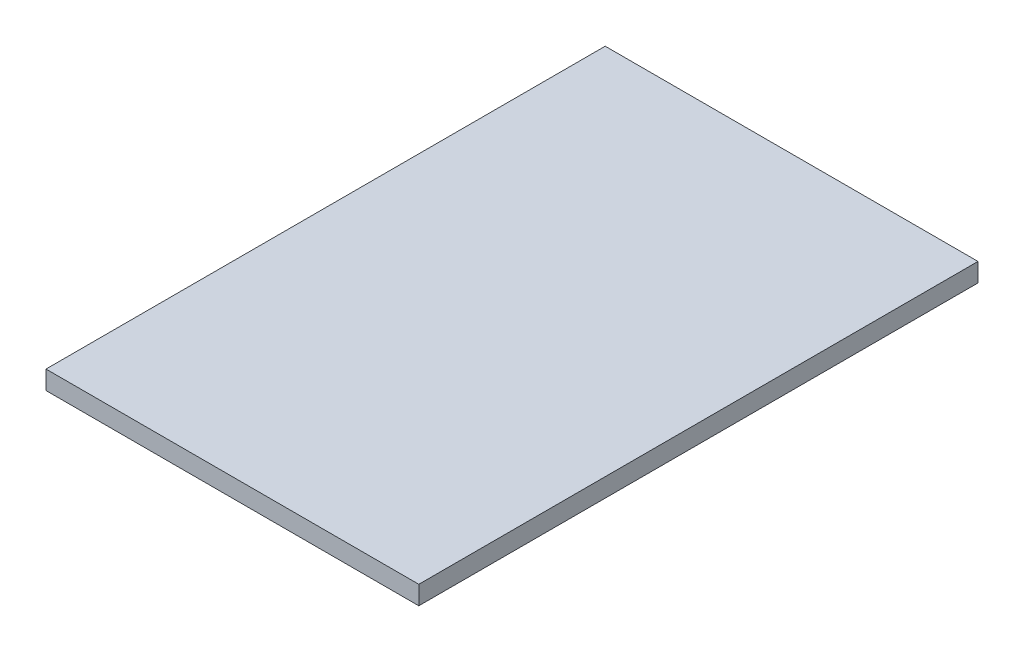
from build123d import *

# Parameters (mm, degrees)
SKETCH2_W           = 200
SKETCH2_H           = 300
BOSS_EXTRUDE1_DEPTH = 10


with BuildPart() as part:
    # Sketch2 → Boss-Extrude1 (new body)
    with BuildSketch(Plane(origin=(0, 0, 0), x_dir=(1, 0, 0), z_dir=(0, 1, 0))):
        Rectangle(SKETCH2_W, SKETCH2_H)
    extrude(amount=BOSS_EXTRUDE1_DEPTH)


solid = part.part
